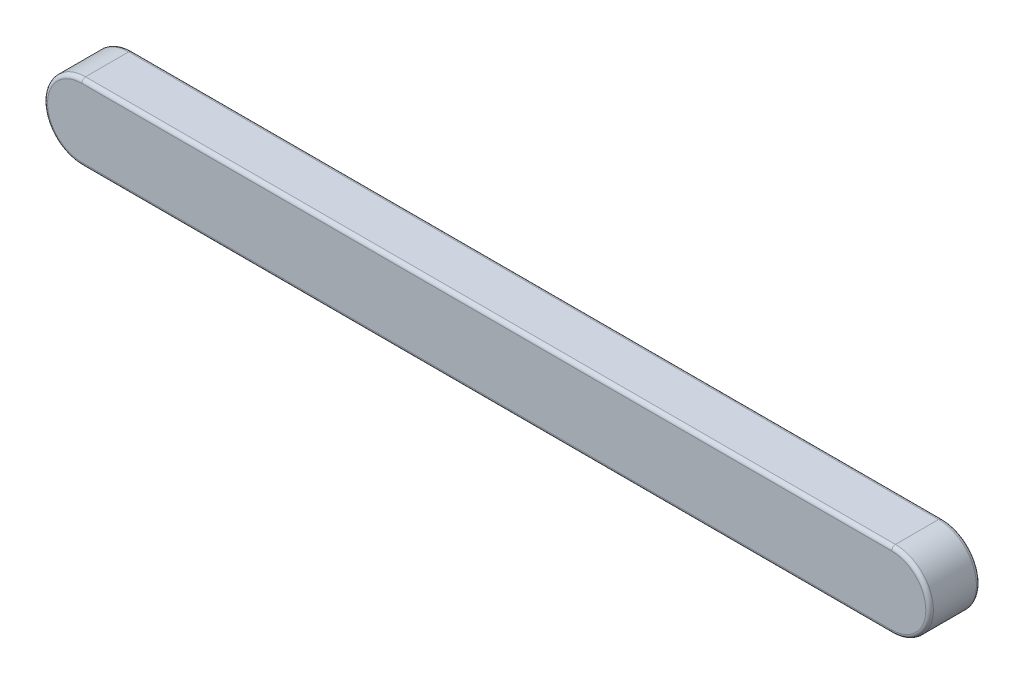
from build123d import *

# Parameters (mm, degrees)
EXTRUDE_523_DEPTH = 8
FILLET_1_R        = 0.6


with BuildPart() as part:
    # 草图1 → Extrude 523 (new body)
    with BuildSketch(Plane.XY):
        with BuildLine():
            Line((-64, 6), (64, 6))
            ThreePointArc((64, 6), (70, 0), (64, -6))
            Line((64, -6), (-64, -6))
            ThreePointArc((-64, -6), (-70, 0), (-64, 6))
        make_face()
    extrude(amount=EXTRUDE_523_DEPTH)

    # 圆角1
    fillet_1_edges = [part.edges().sort_by_distance(p)[0] for p in [
        (70, 0, 8),
        (0, 6, 8),
        (-70, 0, 8),
        (0, 6, 0),
        (70, 0, 0),
        (0, -6, 0),
        (-70, 0, 0),
        (0, -6, 8),
    ]]
    fillet(fillet_1_edges, radius=FILLET_1_R)


solid = part.part
